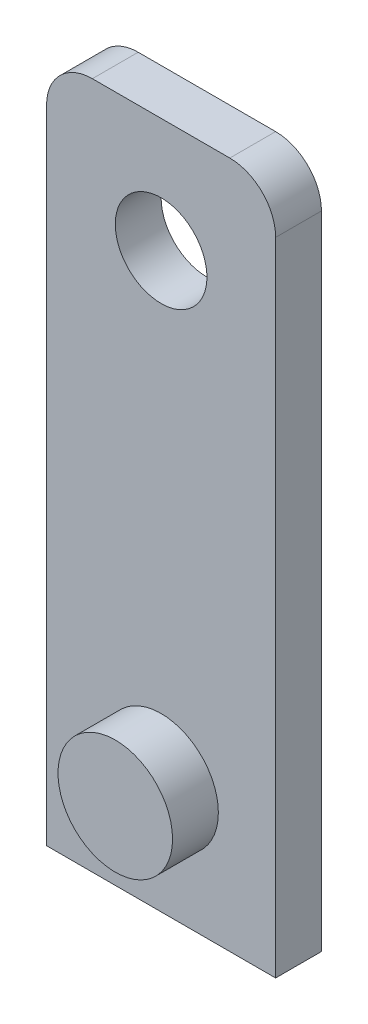
SolidWorks part; units mm, degrees
ref_plane "前视基准面" through (0, 0, 0) normal (0, 0, 1) x (1, 0, 0)
ref_plane "上视基准面" through (0, 0, 0) normal (0, 1, 0) x (1, 0, 0)
ref_plane "右视基准面" through (0, 0, 0) normal (1, 0, 0) x (0, 0, -1)
other "Configuration Table"
sketch "草图1" plane through (0, 0, 0) normal (0, 0, 1) x (1, 0, 0)
  circle A0 centre (0, 0) radius 25
  dimension "D1" = 50
extrude "凸台-拉伸1" add sketch "草图1" along normal blind 20 contours A0
sketch "草图2" plane through (0, 0, 0) normal (0, 0, -1) x (-1, 0, 0)
  line L1 (-50, 250) -> (50, 250)
  line L2 (-50, 250) -> (-50, -50)
  line L3 (-50, -50) -> (50, -50)
  line L4 (50, 250) -> (50, -50)
  line L5 (-50, 250) -> (50, -50) construction
  line L6 (-50, -50) -> (50, 250) construction
  circle A0 centre (0, 200) radius 20
  point P0 (0, 100)
  point P5 (0, 0)
  point P9 (0, 0)
  dimension "D5" = 40
  dimension "D1" = 50
  dimension "D2" = 100
  dimension "D3" = 300
  dimension "D4" = 200
extrude "凸台-拉伸2" add sketch "草图2" along normal blind 20
fillet "圆角1" radius 20 2 edges at (-50, 250, -10) (50, 250, -10)
